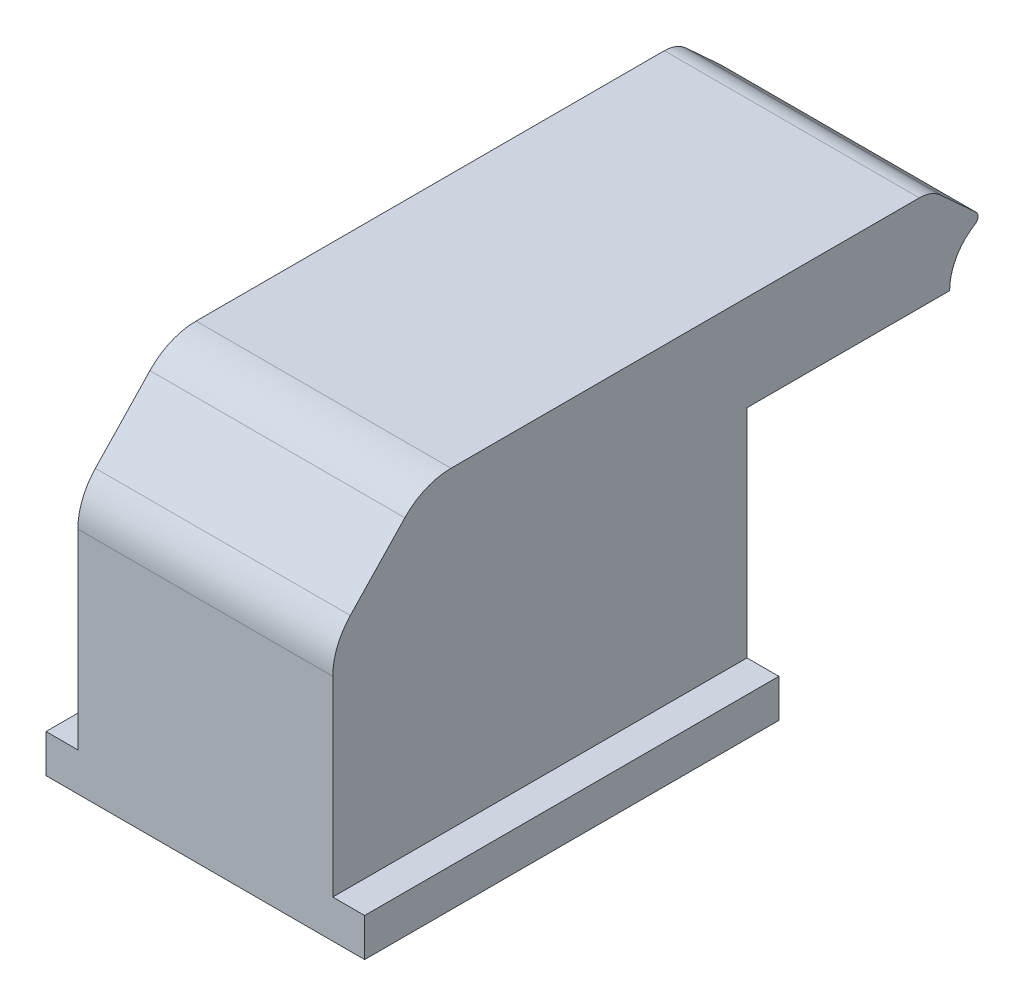
from build123d import *

# Parameters (mm, degrees)
SKETCH1_W           = 50
SKETCH1_H           = 65
BOSS_EXTRUDE1_DEPTH = 6
SKETCH2_W           = 40
SKETCH2_H           = 65
BOSS_EXTRUDE2_DEPTH = 34
SKETCH3_R           = 10.5
CUT_EXTRUDE1_DEPTH  = 47
BOSS_EXTRUDE3_DEPTH = 20
FILLET1_R           = 10


with BuildPart() as part:
    # Sketch1 → Boss-Extrude1 (new body)
    with BuildSketch(Plane(origin=(0, 0, 0), x_dir=(1, 0, 0), z_dir=(0, 1, 0))):
        Rectangle(SKETCH1_W, SKETCH1_H)
    extrude(amount=BOSS_EXTRUDE1_DEPTH)

    # Sketch2 → Boss-Extrude2 (add)
    with BuildSketch(Plane(origin=(0, 6, 0), x_dir=(1, 0, 0), z_dir=(0, 1, 0))):
        Rectangle(SKETCH2_W, SKETCH2_H)
    extrude(amount=BOSS_EXTRUDE2_DEPTH)

    # Sketch3 → Cut-Extrude1 (cut)
    with BuildSketch(Plane(origin=(0, 0, -32.5), x_dir=(-1, 0, 0), z_dir=(0, 0, -1))):
        with Locations((0, 25)):
            Circle(SKETCH3_R)
    extrude(amount=-CUT_EXTRUDE1_DEPTH, mode=Mode.SUBTRACT)

    # Sketch4 → Boss-Extrude3 (add, symmetric)
    with BuildSketch(Plane(origin=(0, 0, 0), x_dir=(0, 0, -1), z_dir=(1, 0, 0))):
        with BuildLine():
            Line((-32.5, 40), (64.3, 40))
            ThreePointArc((64.3, 40), (65.360101389, 44.032598148), (68.266304348, 47.022522419))
            ThreePointArc((68.266304348, 47.022522419), (68.744948846, 47.778544361), (68.426967918, 48.614940117))
            Line((68.426967918, 48.614940117), (62.920069424, 53.680062627))
            ThreePointArc((62.920069424, 53.680062627), (61.351776951, 54.658342685), (59.535229833, 55))
            Line((59.535229833, 55), (28.36278807, 55))
            Line((28.36278807, 55), (-18.236030661, 55))
            Line((-18.236030661, 55), (-32.5, 40))
        make_face()
    extrude(amount=BOSS_EXTRUDE3_DEPTH, both=True)

    # Fillet1
    fillet1_edges = [part.edges().sort_by_distance(p)[0] for p in [
        (0, 40, 32.5),
        (0, 55, 18.236030661),
    ]]
    fillet(fillet1_edges, radius=FILLET1_R)


solid = part.part
